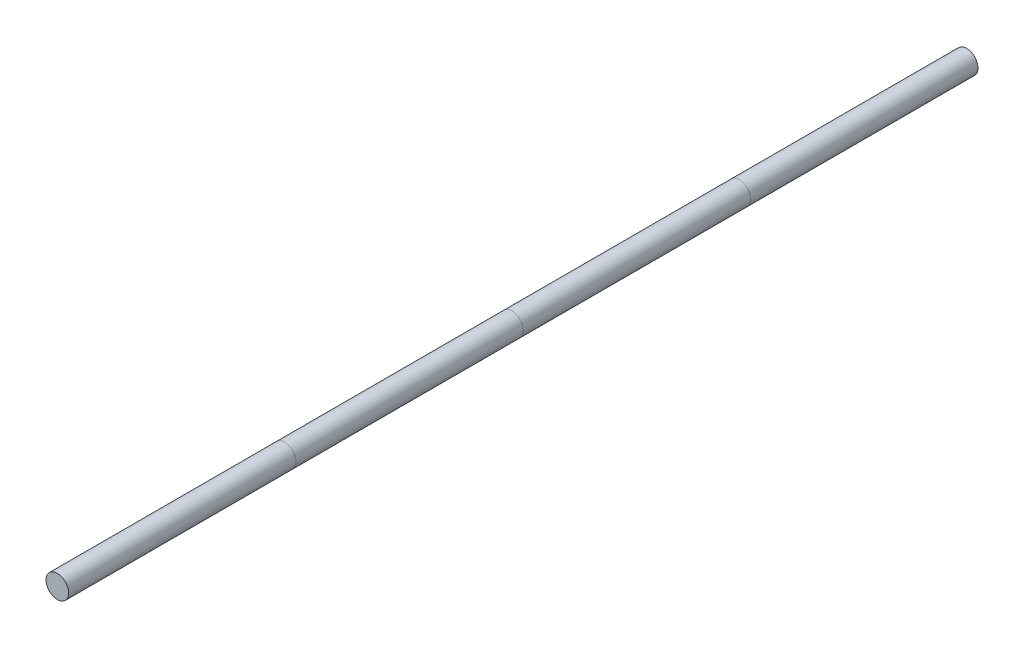
SolidWorks part; units mm, degrees
material "316L"
ref_plane "Front Plane" through (0, 0, 0) normal (0, 0, 1) x (1, 0, 0)
ref_plane "Top Plane" through (0, 0, 0) normal (0, 1, 0) x (1, 0, 0)
ref_plane "Right Plane" through (0, 0, 0) normal (1, 0, 0) x (0, 0, -1)
sketch "Sketch1" plane through (0, 0, 0) normal (0, 0, 1) x (1, 0, 0)
  circle A0 centre (0, 0) radius 5
  dimension "D1" = 10
extrude "Boss-Extrude1" add sketch "Sketch1" along normal blind 400
sketch "Sketch2" plane through (0, 0, 0) normal (0, 1, 0) x (1, 0, 0)
  line L0 (-5, -300) -> (5, -300)
  line L1 (-5, 0) -> (-5, -400) construction
  line L2 (5, -400) -> (5, 0) construction
  line L3 (-5, -400) -> (5, -400) construction
  line L4 (-5, -200) -> (5, -200)
  line L5 (-5, -100) -> (5, -100)
split line "Split Line1"
equation "\"D2@Sketch2\"=\"D1@Sketch2\""
equation "\"D3@Sketch2\"=\"D1@Sketch2\""
